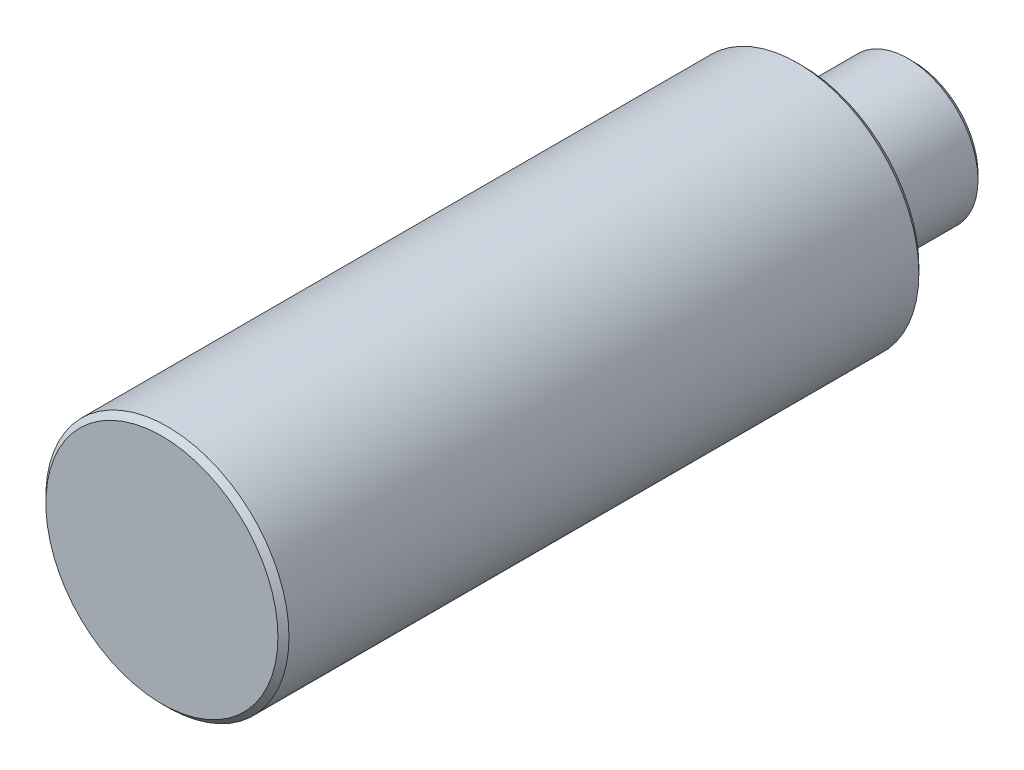
SolidWorks part; units mm, degrees
material "Q235B"
ref_plane "Front Plane" through (0, 0, 0) normal (0, 0, 1) x (1, 0, 0)
ref_plane "Top Plane" through (0, 0, 0) normal (0, 1, 0) x (1, 0, 0)
ref_plane "Right Plane" through (0, 0, 0) normal (1, 0, 0) x (0, 0, -1)
sketch "Sketch1" plane through (0, 0, 0) normal (0, 0, 1) x (1, 0, 0)
  circle A0 centre (0, 0) radius 6.35
  dimension "D1" = 12.7
extrude "Boss-Extrude1" add sketch "Sketch1" along normal blind 10
sketch "Sketch2" plane through (0, 0, 10) normal (0, 0, 1) x (1, 0, 0)
  circle A0 centre (0, 0) radius 11
  dimension "D1" = 22
extrude "Boss-Extrude2" add sketch "Sketch2" along normal blind 58
chamfer "Chamfer1" distance 0.5 angle 45 3 edges at (11, 0, 10) (11, 0, 68) (6.35, 0, 0)
